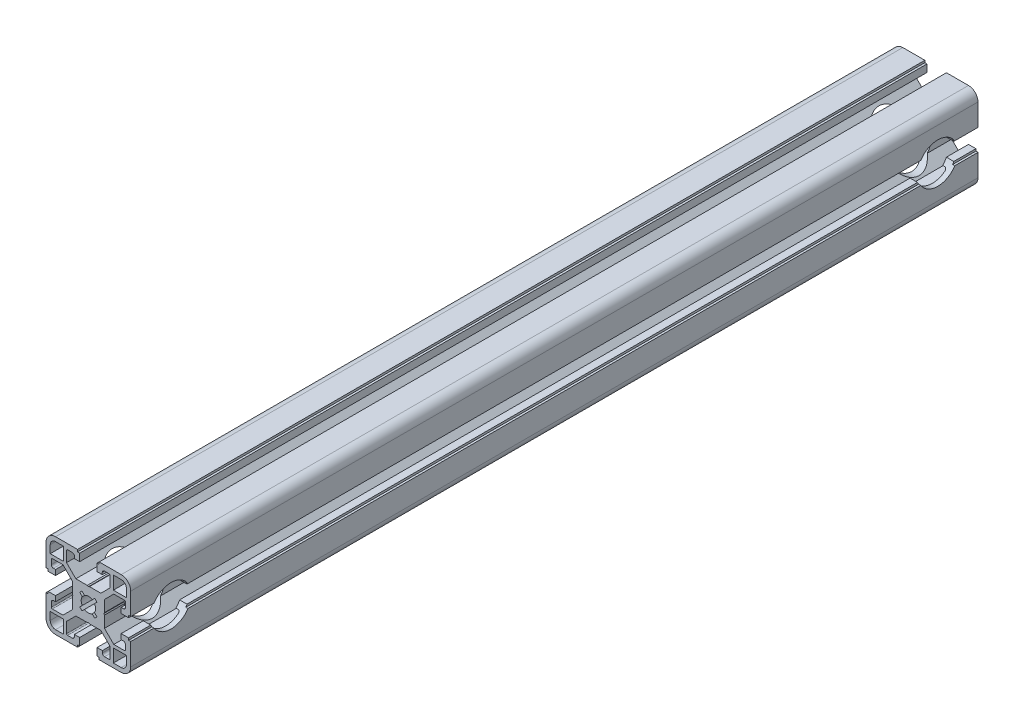
from build123d import *

# Parameters (mm, degrees)
EXTRUDE_1_DEPTH         = 400
HOLE_WIZARD_19_0_19_1_D = 19


with BuildPart() as part:
    # 草图1 → 凸台-拉伸1 (new body)
    with BuildSketch(Plane.XY):
        with BuildLine():
            Line((-18.9995, -4.100341675), (-18.9995, -5.100341675))
            Line((-18.9995, -5.100341675), (-19.9995, -5.100341675))
            Line((-19.9995, -5.100341675), (-19.9995, -15.500341675))
            ThreePointArc((-19.9995, -15.500341675), (-18.681480515, -18.682322191), (-15.4995, -20.000341675))
            Line((-15.4995, -20.000341675), (-5.0995, -20.000341675))
            Line((-5.0995, -20.000341675), (-5.0995, -19.000341675))
            Line((-5.0995, -19.000341675), (-4.0995, -19.000341675))
            Line((-4.0995, -19.000341675), (-4.0995, -15.500341675))
            Line((-4.0995, -15.500341675), (-6.5995, -15.500341675))
            Line((-6.5995, -15.500341675), (-6.5995, -16.500341675))
            ThreePointArc((-6.5995, -16.500341675), (-6.892393219, -17.207448457), (-7.5995, -17.500341675))
            Line((-7.5995, -17.500341675), (-9.7995, -17.500341675))
            ThreePointArc((-9.7995, -17.500341675), (-10.153053391, -17.353895066), (-10.2995, -17.000341675))
            Line((-10.2995, -17.000341675), (-10.2995, -11.997341675))
            Line((-10.2995, -11.997341675), (-5.9025, -7.600341675))
            Line((-5.9025, -7.600341675), (-0.5195, -7.600341675))
            Line((-0.5195, -7.600341675), (0.0005, -7.300341675))
            Line((0.0005, -7.300341675), (0.5195, -7.600341675))
            Line((0.5195, -7.600341675), (5.9035, -7.600341675))
            Line((5.9035, -7.600341675), (10.3005, -11.997341675))
            Line((10.3005, -11.997341675), (10.3005, -17.000341675))
            ThreePointArc((10.3005, -17.000341675), (10.154053391, -17.353895066), (9.8005, -17.500341675))
            Line((9.8005, -17.500341675), (7.6005, -17.500341675))
            ThreePointArc((7.6005, -17.500341675), (6.893393219, -17.207448457), (6.6005, -16.500341675))
            Line((6.6005, -16.500341675), (6.6005, -15.500341675))
            Line((6.6005, -15.500341675), (4.1005, -15.500341675))
            Line((4.1005, -15.500341675), (4.1005, -19.000341675))
            Line((4.1005, -19.000341675), (5.1005, -19.000341675))
            Line((5.1005, -19.000341675), (5.1005, -20.000341675))
            Line((5.1005, -20.000341675), (15.5005, -20.000341675))
            ThreePointArc((15.5005, -20.000341675), (18.682480515, -18.682322191), (20.0005, -15.500341675))
            Line((20.0005, -15.500341675), (20.0005, -5.100341675))
            Line((20.0005, -5.100341675), (19.0005, -5.100341675))
            Line((19.0005, -5.100341675), (19.0005, -4.100341675))
            Line((19.0005, -4.100341675), (15.5005, -4.100341675))
            Line((15.5005, -4.100341675), (15.5005, -6.600341675))
            Line((15.5005, -6.600341675), (16.5005, -6.600341675))
            ThreePointArc((16.5005, -6.600341675), (17.207606781, -6.893234894), (17.5005, -7.600341675))
            Line((17.5005, -7.600341675), (17.5005, -9.800341675))
            ThreePointArc((17.5005, -9.800341675), (17.354053391, -10.153895066), (17.0005, -10.300341675))
            Line((17.0005, -10.300341675), (11.9975, -10.300341675))
            Line((11.9975, -10.300341675), (7.6005, -5.903341675))
            Line((7.6005, -5.903341675), (7.6005, -0.520341675))
            Line((7.6005, -0.520341675), (7.3005, -0.000341675))
            Line((7.3005, -0.000341675), (7.6005, 0.519658325))
            Line((7.6005, 0.519658325), (7.6005, 5.902658325))
            Line((7.6005, 5.902658325), (11.9975, 10.299658325))
            Line((11.9975, 10.299658325), (17.0005, 10.299658325))
            ThreePointArc((17.0005, 10.299658325), (17.354053391, 10.153211715), (17.5005, 9.799658325))
            Line((17.5005, 9.799658325), (17.5005, 7.599658325))
            ThreePointArc((17.5005, 7.599658325), (17.207606781, 6.892551543), (16.5005, 6.599658325))
            Line((16.5005, 6.599658325), (15.5005, 6.599658325))
            Line((15.5005, 6.599658325), (15.5005, 4.099658325))
            Line((15.5005, 4.099658325), (19.0005, 4.099658325))
            Line((19.0005, 4.099658325), (19.0005, 5.099658325))
            Line((19.0005, 5.099658325), (20.0005, 5.099658325))
            Line((20.0005, 5.099658325), (20.0005, 15.499658325))
            ThreePointArc((20.0005, 15.499658325), (18.682480515, 18.68163884), (15.5005, 19.999658325))
            Line((15.5005, 19.999658325), (5.1005, 19.999658325))
            Line((5.1005, 19.999658325), (5.1005, 18.999658325))
            Line((5.1005, 18.999658325), (4.1005, 18.999658325))
            Line((4.1005, 18.999658325), (4.1005, 15.499658325))
            Line((4.1005, 15.499658325), (6.6005, 15.499658325))
            ThreePointArc((6.6005, 15.499658325), (6.393348977, 15.999658325), (6.6005, 16.499658325))
            ThreePointArc((6.6005, 16.499658325), (6.893393219, 17.206765106), (7.6005, 17.499658325))
            Line((7.6005, 17.499658325), (9.8005, 17.499658325))
            ThreePointArc((9.8005, 17.499658325), (10.154053391, 17.353211715), (10.3005, 16.999658325))
            Line((10.3005, 16.999658325), (10.3005, 11.996658325))
            Line((10.3005, 11.996658325), (5.9035, 7.599658325))
            Line((5.9035, 7.599658325), (0.5195, 7.599658325))
            Line((0.5195, 7.599658325), (0.0005, 7.299658325))
            Line((0.0005, 7.299658325), (-0.5195, 7.599658325))
            Line((-0.5195, 7.599658325), (-5.9025, 7.599658325))
            Line((-5.9025, 7.599658325), (-10.2995, 11.996658325))
            Line((-10.2995, 11.996658325), (-10.2995, 16.999658325))
            ThreePointArc((-10.2995, 16.999658325), (-10.153053391, 17.353211715), (-9.7995, 17.499658325))
            Line((-9.7995, 17.499658325), (-7.5995, 17.499658325))
            ThreePointArc((-7.5995, 17.499658325), (-6.892393219, 17.206765106), (-6.5995, 16.499658325))
            Line((-6.5995, 16.499658325), (-6.5995, 15.499658325))
            Line((-6.5995, 15.499658325), (-4.0995, 15.499658325))
            Line((-4.0995, 15.499658325), (-4.0995, 18.999658325))
            Line((-4.0995, 18.999658325), (-5.0995, 18.999658325))
            Line((-5.0995, 18.999658325), (-5.0995, 19.999658325))
            Line((-5.0995, 19.999658325), (-15.4995, 19.999658325))
            ThreePointArc((-15.4995, 19.999658325), (-18.681480515, 18.68163884), (-19.9995, 15.499658325))
            Line((-19.9995, 15.499658325), (-19.9995, 5.099658325))
            Line((-19.9995, 5.099658325), (-18.9995, 5.099658325))
            Line((-18.9995, 5.099658325), (-18.9995, 4.099658325))
            Line((-18.9995, 4.099658325), (-15.4995, 4.099658325))
            Line((-15.4995, 4.099658325), (-15.4995, 6.599658325))
            Line((-15.4995, 6.599658325), (-16.4995, 6.599658325))
            ThreePointArc((-16.4995, 6.599658325), (-17.206606781, 6.892551543), (-17.4995, 7.599658325))
            Line((-17.4995, 7.599658325), (-17.4995, 9.799658325))
            ThreePointArc((-17.4995, 9.799658325), (-17.353053391, 10.153211715), (-16.9995, 10.299658325))
            Line((-16.9995, 10.299658325), (-11.9965, 10.299658325))
            Line((-11.9965, 10.299658325), (-7.5995, 5.902658325))
            Line((-7.5995, 5.902658325), (-7.5995, 0.519658325))
            Line((-7.5995, 0.519658325), (-7.2995, -0.000341675))
            Line((-7.2995, -0.000341675), (-7.5995, -0.520341675))
            Line((-7.5995, -0.520341675), (-7.5995, -5.903341675))
            Line((-7.5995, -5.903341675), (-11.9965, -10.300341675))
            Line((-11.9965, -10.300341675), (-16.9995, -10.300341675))
            ThreePointArc((-16.9995, -10.300341675), (-17.353053391, -10.153895066), (-17.4995, -9.800341675))
            Line((-17.4995, -9.800341675), (-17.4995, -7.600341675))
            ThreePointArc((-17.4995, -7.600341675), (-17.206606781, -6.893234894), (-16.4995, -6.600341675))
            Line((-16.4995, -6.600341675), (-15.4995, -6.600341675))
            Line((-15.4995, -6.600341675), (-15.4995, -4.100341675))
            Line((-15.4995, -4.100341675), (-18.9995, -4.100341675))
        make_face()
        with BuildLine():
            Line((15.5005, -18.000341675), (11.8005, -18.000341675))
            Line((11.8005, -18.000341675), (11.8005, -11.800341675))
            Line((11.8005, -11.800341675), (18.0005, -11.800341675))
            Line((18.0005, -11.800341675), (18.0005, -15.500341675))
            ThreePointArc((18.0005, -15.500341675), (17.268266953, -17.268108628), (15.5005, -18.000341675))
        make_face(mode=Mode.SUBTRACT)
        with BuildLine():
            Line((18.0005, 11.799658325), (11.8005, 11.799658325))
            Line((11.8005, 11.799658325), (11.8005, 17.999658325))
            Line((11.8005, 17.999658325), (15.5005, 17.999658325))
            ThreePointArc((15.5005, 17.999658325), (17.268266953, 17.267425278), (18.0005, 15.499658325))
            Line((18.0005, 15.499658325), (18.0005, 11.799658325))
        make_face(mode=Mode.SUBTRACT)
        with BuildLine():
            Line((-1.8145, -2.875341675), (-3.004391671, -4.066450004))
            Line((-3.004391671, -4.066450004), (-4.065608329, -3.005233346))
            Line((-4.065608329, -3.005233346), (-2.8745, -1.815341675))
            ThreePointArc((-2.8745, -1.815341675), (-3.399473913, -0.000341675), (-2.8745, 1.814658325))
            Line((-2.8745, 1.814658325), (-4.064391671, 3.005766654))
            Line((-4.064391671, 3.005766654), (-3.004391671, 4.065766654))
            Line((-3.004391671, 4.065766654), (-1.8145, 2.874658325))
            ThreePointArc((-1.8145, 2.874658325), (0, 3.399316649), (1.8145, 2.874658325))
            Line((1.8145, 2.874658325), (3.0055, 4.065658325))
            Line((3.0055, 4.065658325), (4.066608329, 3.004549996))
            Line((4.066608329, 3.004549996), (2.8755, 1.814658325))
            ThreePointArc((2.8755, 1.814658325), (3.400473913, -0.000341675), (2.8755, -1.815341675))
            Line((2.8755, -1.815341675), (4.066608329, -3.005233346))
            Line((4.066608329, -3.005233346), (3.0055, -4.066341675))
            Line((3.0055, -4.066341675), (1.8145, -2.875341675))
            ThreePointArc((1.8145, -2.875341675), (0, -3.4), (-1.8145, -2.875341675))
        make_face(mode=Mode.SUBTRACT)
        with BuildLine():
            Line((-17.9995, -15.500341675), (-17.9995, -11.800341675))
            Line((-17.9995, -11.800341675), (-11.7995, -11.800341675))
            Line((-11.7995, -11.800341675), (-11.7995, -18.000341675))
            Line((-11.7995, -18.000341675), (-15.4995, -18.000341675))
            ThreePointArc((-15.4995, -18.000341675), (-17.267266953, -17.268108628), (-17.9995, -15.500341675))
        make_face(mode=Mode.SUBTRACT)
        with BuildLine():
            Line((-11.7995, 17.999658325), (-11.7995, 11.799658325))
            Line((-11.7995, 11.799658325), (-17.9995, 11.799658325))
            Line((-17.9995, 11.799658325), (-17.9995, 15.499658325))
            ThreePointArc((-17.9995, 15.499658325), (-17.267266953, 17.267425278), (-15.4995, 17.999658325))
            Line((-15.4995, 17.999658325), (-11.7995, 17.999658325))
        make_face(mode=Mode.SUBTRACT)
    extrude(amount=-EXTRUDE_1_DEPTH)

    # Ø19.0 (19) 直径孔1 (through all)
    with Locations(Plane(origin=(20.0005, 0, 0), x_dir=(0, 0, -1), z_dir=(1, 0, 0))):
        with Locations((381, -0.000341675), (19, -0.000341675)):
            Hole(HOLE_WIZARD_19_0_19_1_D / 2)


solid = part.part
